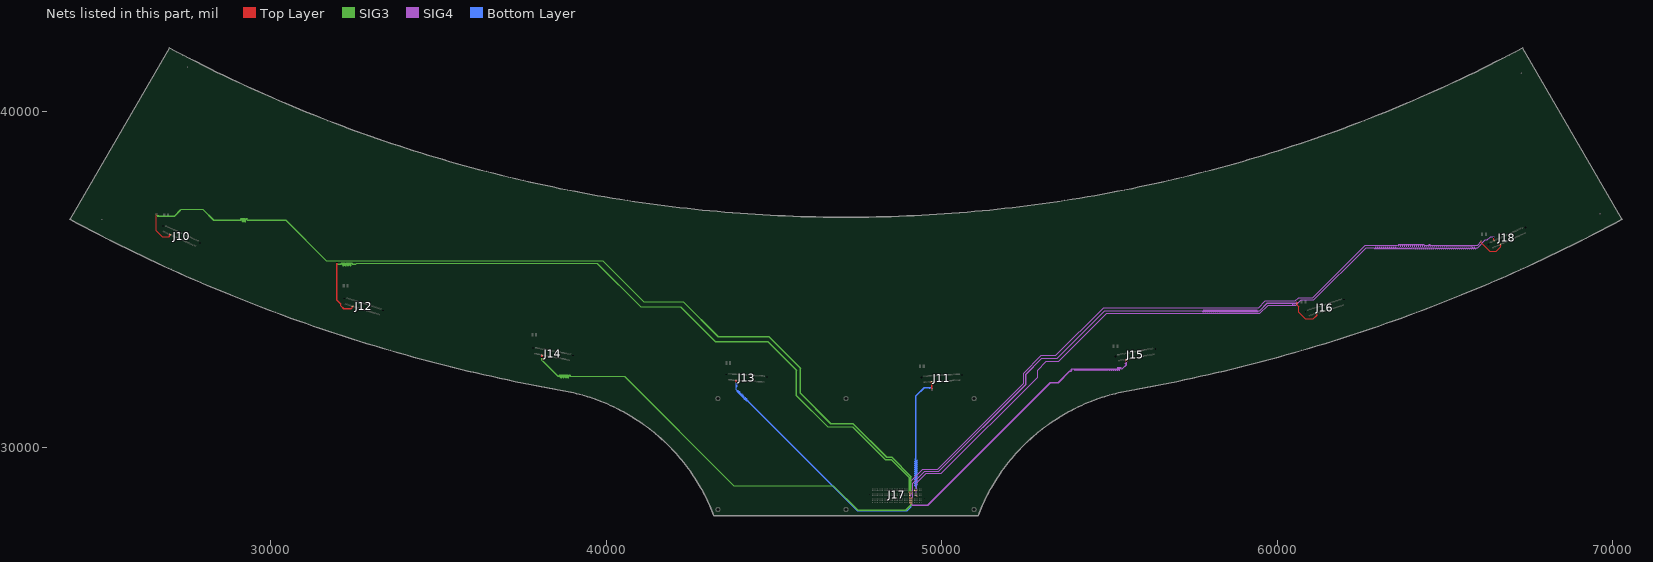
[diagram p0: the nets of this part, all layers, seen from the top]
# Altium PCB MISC86329.PcbDoc (part 3 of 11)
Units mil, origin at the board's own origin, x right, y up, seen from the top; angles counter-clockwise.
Board outline 46247.15 x 13937.21 mil, 6 copper layers (Top Layer, GND2, SIG3, SIG4, POWER5, Bottom Layer); 17 components, 210 nets, 908 pads, 1109 vias.

## Via types
v1: diameter 24, hole 12, Top Layer to Bottom Layer, 684 vias
v2: diameter 18, hole 9, Top Layer to Bottom Layer, 425 vias

## Nets (pads, with @x,y where several pads share a name; then routed paths per layer and width w, separated by ;. In a path a pad name is that pad's centre, name@x,y a point inside that pad or via, vN(x,y) a via of type N, cw(c..) or ccw(c..) an arc to the next point about the centre after c; other vN are vias at no path point) (continued)
DATAIN0P_CH7: J17.E4 J18.10 | length 23895.7
  Top Layer w5: J17.E4@49237.89,28568.8 v2(49261.69,28545) ; v2(66447.5,36256) 66454,36249.5 66454,36196.31 66459.31,36191 J18.10@66459.31,36164.1
  SIG4 w5: v2(49261.69,28545) 49241.69,28565 49241.69,28940.55 49534.14,29233 49992.14,29233 52860,32100.86 52860,32310 53122,32572 53491.14,32572 54914.14,33995 59484.14,33995 59729.14,34240 60552.14,34240 60712.14,34400 61087.14,34400 62648.14,35961 62884.43,35961 62889,35956.43 62889,35941.43 62899.43,35931 62918.57,35931 62929,35941.43 62929,35986.43 62933.57,35991 62944.43,35991 62949,35986.43 62949,35941.43 62959.43,35931 62978.57,35931 62989,35941.43 62989,35986.43 62993.57,35991 63004.43,35991 63009,35986.43 63009,35941.43 63019.43,35931 63038.57,35931 63049,35941.43 63049,35986.43 63053.57,35991 63064.43,35991 63069,35986.43 63069,35941.43 63079.43,35931 63098.57,35931 63109,35941.43 63109,35986.43 63113.57,35991 63124.43,35991 63129,35986.43 63129,35941.43 63139.43,35931 63158.57,35931 63169,35941.43 63169,35986.43 63173.57,35991 63184.43,35991 63189,35986.43 63189,35941.43 63199.43,35931 63218.57,35931 63229,35941.43 63229,35986.43 63233.57,35991 63244.43,35991 63249,35986.43 63249,35941.43 63259.43,35931 63278.57,35931 63289,35941.43 63289,35986.43 63293.57,35991 63304.43,35991 63309,35986.43 63309,35941.43 63319.43,35931 63338.57,35931 63349,35941.43 63349,35986.43 63353.57,35991 63364.43,35991 63369,35986.43 63369,35941.43 63379.43,35931 63398.57,35931 63409,35941.43 63409,35986.43 63413.57,35991 63424.43,35991 63429,35986.43 63429,35941.43 63439.43,35931 63458.57,35931 63469,35941.43 63469,35986.43 63473.57,35991 63484.43,35991 63489,35986.43 63489,35941.43 63499.43,35931 63518.57,35931 63529,35941.43 63529,35986.43 63533.57,35991 63544.43,35991 63549,35986.43 63549,35941.43 63559.43,35931 63578.57,35931 63589,35941.43 63589,35956.43 63593.57,35961 63604.43,35961 63609,35956.43 63609,35941.43 63619.43,35931 63638.57,35931 63649,35941.43 63649,35956.43 63653.57,35961 63664.43,35961 63669,35956.43 63669,35941.43 63679.43,35931 63698.57,35931 63709,35941.43 63709,35956.43 63713.57,35961 63724.43,35961 63729,35956.43 63729,35941.43 63739.43,35931 63758.57,35931 63769,35941.43 63769,35956.43 63773.57,35961 63784.43,35961 63789,35956.43 63789,35941.43 63799.43,35931 63818.57,35931 63829,35941.43 63829,35956.43 63833.57,35961 63844.43,35961 63849,35956.43 63849,35941.43 63859.43,35931 63878.57,35931 63889,35941.43 63889,35956.43 63893.57,35961 63904.43,35961 63909,35956.43 63909,35941.43 63919.43,35931 63938.57,35931 63949,35941.43 63949,35956.43 63953.57,35961 63964.43,35961 63969,35956.43 63969,35941.43 63979.43,35931 63998.57,35931 64009,35941.43 64009,35956.43 64013.57,35961 64024.43,35961 64029,35956.43 64029,35941.43 64039.43,35931 64058.57,35931 64069,35941.43 64069,35956.43 64073.57,35961 64084.43,35961 64089,35956.43 64089,35941.43 64099.43,35931 64118.57,35931 64129,35941.43 64129,35956.43 64133.57,35961 64144.43,35961 64149,35956.43 64149,35941.43 64159.43,35931 64178.57,35931 64189,35941.43 64189,35956.43 64193.57,35961 64204.43,35961 64209,35956.43 64209,35941.43 64219.43,35931 64238.57,35931 64249,35941.43 64249,35956.43 64253.57,35961 64264.43,35961 64269,35956.43 64269,35941.43 64279.43,35931 64298.57,35931 64309,35941.43 64309,35956.43 64313.57,35961 64324.43,35961 64329,35956.43 64329,35941.43 64339.43,35931 64358.57,35931 64369,35941.43 64369,35956.43 64373.57,35961 64384.43,35961 64389,35956.43 64389,35941.43 64399.43,35931 64418.57,35931 64429,35941.43 64429,35956.43 64433.57,35961 64444.43,35961 64449,35956.43 64449,35941.43 64459.43,35931 64478.57,35931 64489,35941.43 64489,35956.43 64493.57,35961 64504.43,35961 64509,35956.43 64509,35941.43 64519.43,35931 64538.57,35931 64549,35941.43 64549,35956.43 64553.57,35961 64564.43,35961 64569,35956.43 64569,35941.43 64579.43,35931 64598.57,35931 64609,35941.43 64609,35956.43 64613.57,35961 64624.43,35961 64629,35956.43 64629,35941.43 64639.43,35931 64658.57,35931 64669,35941.43 64669,35956.43 64673.57,35961 64684.43,35961 64689,35956.43 64689,35941.43 64699.43,35931 64718.57,35931 64729,35941.43 64729,35956.43 64733.57,35961 64744.43,35961 64749,35956.43 64749,35941.43 64759.43,35931 64778.57,35931 64789,35941.43 64789,35956.43 64793.57,35961 64804.43,35961 64809,35956.43 64809,35941.43 64819.43,35931 64838.57,35931 64849,35941.43 64849,35956.43 64853.57,35961 64864.43,35961 64869,35956.43 64869,35941.43 64879.43,35931 64898.57,35931 64909,35941.43 64909,35956.43 64913.57,35961 64924.43,35961 64929,35956.43 64929,35941.43 64939.43,35931 64958.57,35931 64969,35941.43 64969,35956.43 64973.57,35961 64984.43,35961 64989,35956.43 64989,35941.43 64999.43,35931 65018.57,35931 65029,35941.43 65029,35956.43 65033.57,35961 65044.43,35961 65049,35956.43 65049,35941.43 65059.43,35931 65078.57,35931 65089,35941.43 65089,35956.43 65093.57,35961 65104.43,35961 65109,35956.43 65109,35941.43 65119.43,35931 65138.57,35931 65149,35941.43 65149,35956.43 65153.57,35961 65164.43,35961 65169,35956.43 65169,35941.43 65179.43,35931 65198.57,35931 65209,35941.43 65209,35956.43 65213.57,35961 65224.43,35961 65229,35956.43 65229,35941.43 65239.43,35931 65258.57,35931 65269,35941.43 65269,35956.43 65273.57,35961 65284.43,35961 65289,35956.43 65289,35941.43 65299.43,35931 65318.57,35931 65329,35941.43 65329,35956.43 65333.57,35961 65344.43,35961 65349,35956.43 65349,35941.43 65359.43,35931 65378.57,35931 65389,35941.43 65389,35956.43 65393.57,35961 65404.43,35961 65409,35956.43 65409,35941.43 65419.43,35931 65438.57,35931 65449,35941.43 65449,35956.43 65453.57,35961 65464.43,35961 65469,35956.43 65469,35941.43 65479.43,35931 65498.57,35931 65509,35941.43 65509,35956.43 65513.57,35961 65524.43,35961 65529,35956.43 65529,35941.43 65539.43,35931 65558.57,35931 65569,35941.43 65569,35956.43 65573.57,35961 65584.43,35961 65589,35956.43 65589,35941.43 65599.43,35931 65618.57,35931 65629,35941.43 65629,35956.43 65633.57,35961 65644.43,35961 65649,35956.43 65649,35941.43 65659.43,35931 65678.57,35931 65689,35941.43 65689,35956.43 65693.57,35961 65704.43,35961 65709,35956.43 65709,35941.43 65719.43,35931 65738.57,35931 65749,35941.43 65749,35956.43 65753.57,35961 65764.43,35961 65769,35956.43 65769,35941.43 65779.43,35931 65798.57,35931 65809,35941.43 65809,35986.43 65813.57,35991 65824.43,35991 65829,35986.43 65829,35941.43 65839.43,35931 65858.57,35931 65869,35941.43 65869,35986.43 65873.57,35991 65884.43,35991 65889,35986.43 65889,35941.43 65899.43,35931 65918.57,35931 65929,35941.43 65929,35956.43 65933.57,35961 65966.14,35961 66200.14,36195 66263.14,36195 66354.14,36286 66395,36286 66398,36283 66398,36277.73 66401,36274.73 66415,36274.73 66418,36277.73 66418,36283 66421,36286 66442.86,36286 66455,36273.86 66455,36265 v2@66448,36258
DATAIN1N_CH0: J10.17 J17.G8 | length 28225.1
  Top Layer w5: v2(26587.5,36961) 26594,36954.5 26594,36458.86 26773.86,36279 26978.14,36279 27033.49,36334.35 J10.17@27033.49,36336.19 ; J17.G8@49037.89,28668.8 v2(49061.69,28692.61)
  SIG3 w5: v2(26587.5,36961) 26594,36954.5 26594,36925.86 26621.86,36898 27146.14,36898 27323.57,37075.43 ; 27324.07,37075.93 27323.57,37075.43 ; 27359,37098 27362,37098 ; v2(49061.69,28692.61) 49081.69,28712.61 49081.69,29133.31 48505,29710 48351.86,29710 47345.86,30716 46683.86,30716 45787,31612.86 45787,32360 44841,33306 43332.86,33306 42297.86,34341 41116.86,34341 39896.86,35561 31663.86,35561 30448.86,36776 29307.18,36776 29295.5,36787.68 29295.5,36810.18 29289.68,36816 29276.32,36816 29270.5,36810.18 29270.5,36747.68 29258.82,36736 29237.18,36736 29225.5,36747.68 29225.5,36810.18 29219.68,36816 29206.32,36816 29200.5,36810.18 29200.5,36747.68 29188.82,36736 29167.18,36736 29155.5,36747.68 29155.5,36810.18 29149.68,36816 29136.32,36816 29130.5,36810.18 29130.5,36787.68 29118.82,36776 28298.86,36776 27976.86,37098 27362,37098 ; 27323.57,37075.43 27346.14,37098 27362,37098
DATAIN1N_CH1: J12.17 J17.F8 | length 23094.8
  Top Layer w5: 31975,35509.5 31975,34386.86 32088,34273.86 32088,34219.86 32172.86,34135 32410.14,34135 32442.98,34167.84 32442.98,34187.61 J12.17@32463.01,34207.64 ; J17.F8@49037.89,28618.8 v2(49061.69,28642.61)
  SIG3 w5: v2(31968.5,35516) v2@31971,35516 ; v2@31970,35517 v2@31971,35516 ; v2@31975,35516 v2@31971,35516 ; v2(49061.69,28642.61) 49032,28672.3 49032,29102 48492,29642 48312.86,29642 47341.86,30613 46603.86,30613 45673,31543.86 45673,32302 44819,33156 43248.86,33156 42215.86,34189 41027.86,34189 39728.86,35488 32571.14,35488 32545.14,35462 32441.18,35462 32429.5,35473.68 32429.5,35494.91 32423.68,35500.73 32410.32,35500.73 32404.5,35494.91 32404.5,35434.95 32392.82,35423.27 32371.18,35423.27 32359.5,35434.95 32359.5,35494.91 32353.68,35500.73 32340.32,35500.73 32334.5,35494.91 32334.5,35434.95 32322.82,35423.27 32301.18,35423.27 32289.5,35434.95 32289.5,35494.91 32283.68,35500.73 32270.32,35500.73 32264.5,35494.91 32264.5,35434.95 32252.82,35423.27 32231.18,35423.27 32219.5,35434.95 32219.5,35494.91 32213.68,35500.73 32200.32,35500.73 32194.5,35494.91 32194.5,35434.95 32182.82,35423.27 32161.18,35423.27 32149.5,35434.95 32149.5,35494.91 32143.68,35500.73 32130.32,35500.73 32124.5,35494.91 32124.5,35473.68 32112.82,35462 31999,35462 31975,35486 31975,35512 v2@31971,35516
DATAIN1N_CH2: J14.17 J17.B8 | length 13805.5
  Top Layer w5: v2(38103.5,32687) 38097,32693.5 38097,32728 38110,32741 J14.17@38110,32753 ; J14.17@38111.46,32753 J14.17@38111.46,32756.64 ; J17.B8@49037.89,28418.8 v2(49061.69,28395)
  SIG3 w5: v2@38103,32685 38097,32679 38097,32662.75 38103.25,32656.5 38115.92,32656.5 38122.17,32650.25 38122.17,32637.75 38115.92,32631.5 38103.25,32631.5 38097,32625.25 38097,32599 38568,32128 38598.68,32128 38604.5,32133.82 38604.5,32153.32 38616.18,32165 38637.82,32165 38649.5,32153.32 38649.5,32096.82 38655.32,32091 38668.68,32091 38674.5,32096.82 38674.5,32153.32 38686.18,32165 38707.82,32165 38719.5,32153.32 38719.5,32096.82 38725.32,32091 38738.68,32091 38744.5,32096.82 38744.5,32153.32 38756.18,32165 38777.82,32165 38789.5,32153.32 38789.5,32096.82 38795.32,32091 38808.68,32091 38814.5,32096.82 38814.5,32153.32 38826.18,32165 38847.82,32165 38859.5,32153.32 38859.5,32096.82 38865.32,32091 38878.68,32091 38884.5,32096.82 38884.5,32153.32 38896.18,32165 38917.82,32165 38929.5,32153.32 38929.5,32133.82 38935.32,32128 40551,32128 43810,28869 46771,28869 47499,28141 48933,28141 49081.69,28289.69 49081.69,28375 v2(49061.69,28395)
DATAIN1N_CH3: J13.17 J17.A8 | length 7748.3
  Top Layer w5: 43883.92,31946.5 43883.92,31969.28 43894.64,31980 J13.17@43894.64,32004.84 ; J17.A8@49037.89,28368.8 v2(49061.69,28345)
  Bottom Layer w5: v2@43889,31937 43884,31932 43884,31898.5 43889,31893.5 43896.36,31893.5 43901.36,31888.5 43901.36,31873.5 43896.36,31868.5 43889,31868.5 43884,31863.5 43884,31848.5 43889,31843.5 43896.36,31843.5 43901.36,31838.5 43901.36,31823.5 43896.36,31818.5 43889,31818.5 43884,31813.5 43884,31729 43906.95,31706.05 43911.65,31706.05 43916.95,31711.35 43929.94,31711.35 43941.7,31699.58 43941.7,31686.6 43922.26,31667.15 43922.26,31662.46 43928.17,31656.55 43932.86,31656.55 43952.31,31675.99 43965.29,31675.99 43977.06,31664.23 43977.06,31651.24 43957.61,31631.8 43957.61,31627.1 43963.52,31621.19 43968.22,31621.19 43987.67,31640.64 44000.65,31640.64 44012.41,31628.87 44012.41,31615.89 43992.97,31596.44 43992.97,31591.75 43998.88,31585.84 44003.58,31585.84 44023.02,31605.28 44036,31605.28 44047.77,31593.51 44047.77,31580.53 44028.32,31561.09 44028.32,31556.39 44034.23,31550.48 44038.93,31550.48 44058.38,31569.93 44071.36,31569.93 44083.12,31558.16 44083.12,31545.18 44063.68,31525.73 44063.68,31521.04 44069.59,31515.13 44074.29,31515.13 44093.73,31534.57 44106.71,31534.57 44118.48,31522.8 44118.48,31509.82 44099.03,31490.38 44099.03,31485.68 44104.94,31479.77 44109.64,31479.77 44129.09,31499.22 44142.07,31499.22 44153.84,31487.45 44153.84,31474.47 44134.39,31455.02 44134.39,31450.33 44140.3,31444.42 44145,31444.42 44164.44,31463.86 44177.42,31463.86 44189.19,31452.09 44189.19,31439.11 44169.75,31419.67 44169.75,31414.97 44175.66,31409.06 44180.35,31409.06 44199.8,31428.51 44212.78,31428.51 44224.55,31416.74 44224.55,31403.76 44219.24,31398.45 44219.24,31393.76 47481,28132 48977,28132 49081.69,28236.69 49081.69,28325 v2(49061.69,28345)
  other v2: 43890.42,31940
DATAIN1N_CH4: J11.17 J17.H5 | length 5093.3
  Top Layer w5: J17.H5@49187.89,28718.8 v2(49211.69,28742.61) ; 49715.61,31718.5 49715.61,31927.28 49726.33,31938 J11.17@49726.33,31963.43
  Bottom Layer w5: v2(49211.69,28742.61) 49231.69,28762.61 49231.69,28842.43 49227.12,28847 49212.12,28847 49201.69,28857.43 49201.69,28876.57 49212.12,28887 49257.12,28887 49261.69,28891.57 49261.69,28902.43 49257.12,28907 49212.12,28907 49201.69,28917.43 49201.69,28936.57 49212.12,28947 49257.12,28947 49261.69,28951.57 49261.69,28962.43 49257.12,28967 49212.12,28967 49201.69,28977.43 49201.69,28996.57 49212.12,29007 49257.12,29007 49261.69,29011.57 49261.69,29022.43 49257.12,29027 49212.12,29027 49201.69,29037.43 49201.69,29056.57 49212.12,29067 49257.12,29067 49261.69,29071.57 49261.69,29082.43 49257.12,29087 49212.12,29087 49201.69,29097.43 49201.69,29116.57 49212.12,29127 49257.12,29127 49261.69,29131.57 49261.69,29142.43 49257.12,29147 49212.12,29147 49201.69,29157.43 49201.69,29176.57 49212.12,29187 49257.12,29187 49261.69,29191.57 49261.69,29202.43 49257.12,29207 49212.12,29207 49201.69,29217.43 49201.69,29236.57 49212.12,29247 49257.12,29247 49261.69,29251.57 49261.69,29262.43 49257.12,29267 49212.12,29267 49201.69,29277.43 49201.69,29296.57 49212.12,29307 49257.12,29307 49261.69,29311.57 49261.69,29322.43 49257.12,29327 49212.12,29327 49201.69,29337.43 49201.69,29356.57 49212.12,29367 49257.12,29367 49261.69,29371.57 49261.69,29382.43 49257.12,29387 49212.12,29387 49201.69,29397.43 49201.69,29416.57 49212.12,29427 49257.12,29427 49261.69,29431.57 49261.69,29442.43 49257.12,29447 49212.12,29447 49201.69,29457.43 49201.69,29476.57 49212.12,29487 49257.12,29487 49261.69,29491.57 49261.69,29502.43 49257.12,29507 49212.12,29507 49201.69,29517.43 49201.69,29536.57 49212.12,29547 49257.12,29547 49261.69,29551.57 49261.69,29562.43 49257.12,29567 49212.12,29567 49201.69,29577.43 49201.69,29596.57 49212.12,29607 49257.12,29607 49261.69,29611.57 49261.69,29622.43 49257.12,29627 49227,29627 49214,29640 49214,29669.14 49231.69,29686.83 49231.69,31545.69 49485,31799 49672.14,31799 49716,31755.14 49716,31717 v2@49721,31712
  other v2: 49722.11,31712
DATAIN1N_CH5: J15.17 J17.C8 | length 10127.3
  Top Layer w5: J17.C8@49037.89,28468.8 v2(49061.69,28445) ; v2(55513.5,32564) 55507,32570.5 55507,32594.39 55519.61,32607 J15.17@55519.61,32633.03
  SIG4 w5: v2(49061.69,28445) 49081.69,28425 49081.69,28330.17 49125.86,28286 49595.14,28286 53246.14,31937 53481.14,31937 53822.14,32278 53853.29,32278 ; 53853.32,32277.97 53867.97,32277.97 53880,32290 53880,32307.86 53874.54,32313.32 53874.54,32330.39 53887.14,32343 53946.43,32343 53951,32338.43 53951,32313.43 53961.43,32303 53980.57,32303 53991,32313.43 53991,32338.43 53995.57,32343 54006.43,32343 54011,32338.43 54011,32313.43 54021.43,32303 54040.57,32303 54051,32313.43 54051,32338.43 54055.57,32343 54066.43,32343 54071,32338.43 54071,32313.43 54081.43,32303 54100.57,32303 54111,32313.43 54111,32338.43 54115.57,32343 54126.43,32343 54131,32338.43 54131,32313.43 54141.43,32303 54160.57,32303 54171,32313.43 54171,32338.43 54175.57,32343 54186.43,32343 54191,32338.43 54191,32313.43 54201.43,32303 54220.57,32303 54231,32313.43 54231,32338.43 54235.57,32343 54246.43,32343 54251,32338.43 54251,32313.43 54261.43,32303 54280.57,32303 54291,32313.43 54291,32338.43 54295.57,32343 54306.43,32343 54311,32338.43 54311,32313.43 54321.43,32303 54340.57,32303 54351,32313.43 54351,32338.43 54355.57,32343 54366.43,32343 54371,32338.43 54371,32313.43 54381.43,32303 54400.57,32303 54411,32313.43 54411,32338.43 54415.57,32343 54426.43,32343 54431,32338.43 54431,32313.43 54441.43,32303 54460.57,32303 54471,32313.43 54471,32338.43 54475.57,32343 54486.43,32343 54491,32338.43 54491,32313.43 54501.43,32303 54520.57,32303 54531,32313.43 54531,32338.43 54535.57,32343 54546.43,32343 54551,32338.43 54551,32313.43 54561.43,32303 54580.57,32303 54591,32313.43 54591,32338.43 54595.57,32343 54606.43,32343 54611,32338.43 54611,32313.43 54621.43,32303 54640.57,32303 54651,32313.43 54651,32338.43 54655.57,32343 54666.43,32343 54671,32338.43 54671,32313.43 54681.43,32303 54700.57,32303 54711,32313.43 54711,32338.43 54715.57,32343 54726.43,32343 54731,32338.43 54731,32313.43 54741.43,32303 54760.57,32303 54771,32313.43 54771,32338.43 54775.57,32343 54786.43,32343 54791,32338.43 54791,32313.43 54801.43,32303 54820.57,32303 54831,32313.43 54831,32338.43 54835.57,32343 54846.43,32343 54851,32338.43 54851,32313.43 54861.43,32303 54880.57,32303 54891,32313.43 54891,32338.43 54895.57,32343 54906.43,32343 54911,32338.43 54911,32313.43 54921.43,32303 54940.57,32303 54951,32313.43 54951,32338.43 54955.57,32343 54966.43,32343 54971,32338.43 54971,32313.43 54981.43,32303 55000.57,32303 55011,32313.43 55011,32338.43 55015.57,32343 55026.43,32343 55031,32338.43 55031,32313.43 55041.43,32303 55060.57,32303 55071,32313.43 55071,32338.43 55075.57,32343 55086.43,32343 55091,32338.43 55091,32313.43 55101.43,32303 55120.57,32303 55131,32313.43 55131,32338.43 55135.57,32343 55146.43,32343 55151,32338.43 55151,32313.43 55161.43,32303 55180.57,32303 55191,32313.43 55191,32338.43 55195.57,32343 55206.43,32343 55211,32338.43 55211,32313.43 55221.43,32303 55240.57,32303 55251,32313.43 55251,32378.43 55255.57,32383 55266.43,32383 55271,32378.43 55271,32313.43 55281.43,32303 55300.57,32303 55311,32313.43 55311,32378.43 55315.57,32383 55326.43,32383 55331,32378.43 55331,32353.43 55341.43,32343 55382,32343 55507,32468 55507,32556 v2@55515,32564
DATAIN1N_CH6: J16.17 J17.D8 | length 18293.4
  Top Layer w5: J17.D8@49037.89,28518.8 v2(49061.69,28495) ; 60590,34344.5 60590,34240 60634,34196 60634,34030.86 60832.86,33832 61077.14,33832 61187,33941.86 61187,33975.91 ; 61188.09,33977 J16.17@61188.09,34003.67
  SIG4 w5: v2(49061.69,28495) 49088.36,28495 49104.86,28511.5 49113.5,28511.5 49131,28529 49131,28937 49492,29298 49914,29298 52506,31890 52506,32186.14 52984.86,32665 53444,32665 54860,34081 57770,34081 57783,34068 57783,34055.57 57787.57,34051 57798.43,34051 57803,34055.57 57803,34100.57 57813.43,34111 57832.57,34111 57843,34100.57 57843,34055.57 57847.57,34051 57858.43,34051 57863,34055.57 57863,34100.57 57873.43,34111 57892.57,34111 57903,34100.57 57903,34055.57 57907.57,34051 57918.43,34051 57923,34055.57 57923,34100.57 57933.43,34111 57952.57,34111 57963,34100.57 57963,34055.57 57967.57,34051 57978.43,34051 57983,34055.57 57983,34100.57 57993.43,34111 58012.57,34111 58023,34100.57 58023,34055.57 58027.57,34051 58038.43,34051 58043,34055.57 58043,34100.57 58053.43,34111 58072.57,34111 58083,34100.57 58083,34055.57 58087.57,34051 58098.43,34051 58103,34055.57 58103,34100.57 58113.43,34111 58132.57,34111 58143,34100.57 58143,34055.57 58147.57,34051 58158.43,34051 58163,34055.57 58163,34100.57 58173.43,34111 58192.57,34111 58203,34100.57 58203,34055.57 58207.57,34051 58218.43,34051 58223,34055.57 58223,34100.57 58233.43,34111 58252.57,34111 58263,34100.57 58263,34055.57 58267.57,34051 58278.43,34051 58283,34055.57 58283,34100.57 58293.43,34111 58312.57,34111 58323,34100.57 58323,34055.57 58327.57,34051 58338.43,34051 58343,34055.57 58343,34100.57 58353.43,34111 58372.57,34111 58383,34100.57 58383,34055.57 58387.57,34051 58398.43,34051 58403,34055.57 58403,34100.57 58413.43,34111 58432.57,34111 58443,34100.57 58443,34055.57 58447.57,34051 58458.43,34051 58463,34055.57 58463,34100.57 58473.43,34111 58492.57,34111 58503,34100.57 58503,34055.57 58507.57,34051 58518.43,34051 58523,34055.57 58523,34100.57 58533.43,34111 58552.57,34111 58563,34100.57 58563,34055.57 58567.57,34051 58578.43,34051 58583,34055.57 58583,34100.57 58593.43,34111 58612.57,34111 58623,34100.57 58623,34055.57 58627.57,34051 58638.43,34051 58643,34055.57 58643,34100.57 58653.43,34111 58672.57,34111 58683,34100.57 58683,34055.57 58687.57,34051 58698.43,34051 58703,34055.57 58703,34100.57 58713.43,34111 58732.57,34111 58743,34100.57 58743,34055.57 58747.57,34051 58758.43,34051 58763,34055.57 58763,34100.57 58773.43,34111 58792.57,34111 58803,34100.57 58803,34055.57 58807.57,34051 58818.43,34051 58823,34055.57 58823,34100.57 58833.43,34111 58852.57,34111 58863,34100.57 58863,34055.57 58867.57,34051 58878.43,34051 58883,34055.57 58883,34100.57 58893.43,34111 58912.57,34111 58923,34100.57 58923,34055.57 58927.57,34051 58938.43,34051 58943,34055.57 58943,34100.57 58953.43,34111 58972.57,34111 58983,34100.57 58983,34055.57 58987.57,34051 58998.43,34051 59003,34055.57 59003,34100.57 59013.43,34111 59032.57,34111 59043,34100.57 59043,34055.57 59047.57,34051 59058.43,34051 59063,34055.57 59063,34100.57 59073.43,34111 59092.57,34111 59103,34100.57 59103,34055.57 59107.57,34051 59118.43,34051 59123,34055.57 59123,34100.57 59133.43,34111 59152.57,34111 59163,34100.57 59163,34055.57 59167.57,34051 59178.43,34051 59183,34055.57 59183,34100.57 59193.43,34111 59212.57,34111 59223,34100.57 59223,34055.57 59227.57,34051 59238.43,34051 59243,34055.57 59243,34100.57 59253.43,34111 59272.57,34111 59283,34100.57 59283,34055.57 59287.57,34051 59298.43,34051 59303,34055.57 59303,34100.57 59313.43,34111 59332.57,34111 59343,34100.57 59343,34055.57 59347.57,34051 59358.43,34051 59363,34055.57 59363,34100.57 59373.43,34111 59392.57,34111 59403,34100.57 59403,34055.57 59407.57,34051 59418.43,34051 59423,34055.57 59423,34070.57 59433.43,34081 59472,34081 59699,34308 60564,34308 60590,34334 60590,34346 v2@60584,34352
  other v2: 60583.5,34351
DATAIN1N_CH7: J17.E8 J18.17 | length 23896.2
  Top Layer w5: J17.E8@49037.89,28568.8 v2(49061.69,28545) ; 66083,36150.5 66083,36099.86 66328.86,35854 66531.14,35854 66654,35976.86 66654,36020.63 66647.29,36027.34 J18.17@66647.29,36054.9
  SIG4 w5: v2(49061.69,28545) 49081.69,28565 49081.69,29002.14 49440.55,29361 49888,29361 52438,31911 52438,32218 52965,32745 53404,32745 54828,34169 59448,34169 59647,34368 60538,34368 60636,34466 61051,34466 62619,36034 63576,36034 63599,36011 63612,36011 63621.5,36020.5 63621.5,36053.57 63631.93,36064 63651.07,36064 63661.5,36053.57 63661.5,36008.57 63666.07,36004 63676.93,36004 63681.5,36008.57 63681.5,36053.57 63691.93,36064 63711.07,36064 63721.5,36053.57 63721.5,36008.57 63726.07,36004 63736.93,36004 63741.5,36008.57 63741.5,36053.57 63751.93,36064 63771.07,36064 63781.5,36053.57 63781.5,36008.57 63786.07,36004 63796.93,36004 63801.5,36008.57 63801.5,36053.57 63811.93,36064 63831.07,36064 63841.5,36053.57 63841.5,36008.57 63846.07,36004 63856.93,36004 63861.5,36008.57 63861.5,36053.57 63871.93,36064 63891.07,36064 63901.5,36053.57 63901.5,36008.57 63906.07,36004 63916.93,36004 63921.5,36008.57 63921.5,36053.57 63931.93,36064 63951.07,36064 63961.5,36053.57 63961.5,36008.57 63966.07,36004 63976.93,36004 63981.5,36008.57 63981.5,36053.57 63991.93,36064 64011.07,36064 64021.5,36053.57 64021.5,36008.57 64026.07,36004 64036.93,36004 64041.5,36008.57 64041.5,36053.57 64051.93,36064 64071.07,36064 64081.5,36053.57 64081.5,36008.57 64086.07,36004 64096.93,36004 64101.5,36008.57 64101.5,36053.57 64111.93,36064 64131.07,36064 64141.5,36053.57 64141.5,36008.57 64146.07,36004 64156.93,36004 64161.5,36008.57 64161.5,36053.57 64171.93,36064 64191.07,36064 64201.5,36053.57 64201.5,36008.57 64206.07,36004 64216.93,36004 64221.5,36008.57 64221.5,36053.57 64231.93,36064 64251.07,36064 64261.5,36053.57 64261.5,36008.57 64266.07,36004 64276.93,36004 64281.5,36008.57 64281.5,36053.57 64291.93,36064 64311.07,36064 64321.5,36053.57 64321.5,36008.57 64326.07,36004 64336.93,36004 64341.5,36008.57 64341.5,36053.57 64351.93,36064 64371.07,36064 64381.5,36053.57 64381.5,36008.57 64386.07,36004 64396.93,36004 64401.5,36008.57 64401.5,36023.57 64411.93,36034 64431.07,36034 64441.5,36023.57 64441.5,36008.57 64446.07,36004 64456.93,36004 64461.5,36008.57 64461.5,36023.57 64471.93,36034 64491.07,36034 64501.5,36023.57 64501.5,36008.57 64506.07,36004 64516.93,36004 64521.5,36008.57 64521.5,36053.57 64531.93,36064 64551.07,36064 64561.5,36053.57 64561.5,36008.57 64566.07,36004 64576.93,36004 64581.5,36008.57 64581.5,36023.57 64591.93,36034 64611.07,36034 64621.5,36023.57 64621.5,36008.57 64626.07,36004 64636.93,36004 64641.5,36008.57 64641.5,36023.57 64651.93,36034 64671.07,36034 64681.5,36023.57 64681.5,36008.57 64686.07,36004 64696.93,36004 64701.5,36008.57 64701.5,36023.57 64711.93,36034 64731.07,36034 64741.5,36023.57 64741.5,36008.57 64746.07,36004 64756.93,36004 64761.5,36008.57 64761.5,36023.57 64771.93,36034 64791.07,36034 64801.5,36023.57 64801.5,36008.57 64806.07,36004 64816.93,36004 64821.5,36008.57 64821.5,36023.57 64831.93,36034 64851.07,36034 64861.5,36023.57 64861.5,36008.57 64866.07,36004 64876.93,36004 64881.5,36008.57 64881.5,36023.57 64891.93,36034 64911.07,36034 64921.5,36023.57 64921.5,36008.57 64926.07,36004 64936.93,36004 64941.5,36008.57 64941.5,36023.57 64951.93,36034 64971.07,36034 64981.5,36023.57 64981.5,36008.57 64986.07,36004 64996.93,36004 65001.5,36008.57 65001.5,36023.57 65011.93,36034 65031.07,36034 65041.5,36023.57 65041.5,36008.57 65046.07,36004 65056.93,36004 65061.5,36008.57 65061.5,36023.57 65071.93,36034 65091.07,36034 65101.5,36023.57 65101.5,36008.57 65106.07,36004 65116.93,36004 65121.5,36008.57 65121.5,36023.57 65131.93,36034 65151.07,36034 65161.5,36023.57 65161.5,36008.57 65166.07,36004 65176.93,36004 65181.5,36008.57 65181.5,36023.57 65191.93,36034 65211.07,36034 65221.5,36023.57 65221.5,36008.57 65226.07,36004 65236.93,36004 65241.5,36008.57 65241.5,36023.57 65251.93,36034 65271.07,36034 65281.5,36023.57 65281.5,36008.57 65286.07,36004 65296.93,36004 65301.5,36008.57 65301.5,36023.57 65311.93,36034 65331.07,36034 65341.5,36023.57 65341.5,36008.57 65346.07,36004 65356.93,36004 65361.5,36008.57 65361.5,36023.57 65371.93,36034 65391.07,36034 65401.5,36023.57 65401.5,36008.57 65406.07,36004 65416.93,36004 65421.5,36008.57 65421.5,36023.57 65431.93,36034 65451.07,36034 65461.5,36023.57 65461.5,36008.57 65466.07,36004 65476.93,36004 65481.5,36008.57 65481.5,36023.57 65491.93,36034 65511.07,36034 65521.5,36023.57 65521.5,36008.57 65526.07,36004 65536.93,36004 65541.5,36008.57 65541.5,36023.57 65551.93,36034 65571.07,36034 65581.5,36023.57 65581.5,36008.57 65586.07,36004 65596.93,36004 65601.5,36008.57 65601.5,36023.57 65611.93,36034 65631.07,36034 65641.5,36023.57 65641.5,36008.57 65646.07,36004 65656.93,36004 65661.5,36008.57 65661.5,36023.57 65671.93,36034 65691.07,36034 65701.5,36023.57 65701.5,36008.57 65706.07,36004 65716.93,36004 65721.5,36008.57 65721.5,36023.57 65731.93,36034 65751.07,36034 65761.5,36023.57 65761.5,36008.57 65766.07,36004 65776.93,36004 65781.5,36008.57 65781.5,36023.57 65791.93,36034 65975.86,36034 66083,36141.14 66083,36151 v2@66079,36155
  other v2: 66076.5,36157
DATAIN1P_CH0: J10.15 J17.G7 | length 28224.5
  Top Layer w5: v2(26610.5,36961) 26604,36954.5 26604,36463 26778,36289 26974,36289 27004.85,36319.85 J10.15@27004.85,36349.28 ; J17.G7@49087.89,28668.8 v2(49111.69,28692.61)
  SIG3 w5: v2(26610.5,36961) 26604,36954.5 26604,36930 26626,36908 26652,36908 26657,36913 26657,36921.38 26662,36926.38 26672,36926.38 26677,36921.38 26677,36913 26682,36908 27142,36908 27315,37081 ; 27317,37083 27315,37081 ; 27359,37108 27362,37108 ; v2(49111.69,28692.61) 49091.69,28712.61 49091.69,29137.45 48509.14,29720 48356,29720 47350,30726 46688,30726 45797,31617 45797,32364.14 44845.14,33316 43337,33316 42302,34351 41121,34351 39901,35571 31668,35571 30453,36786 29311.32,36786 29305.5,36791.82 29305.5,36814.32 29293.82,36826 29272.18,36826 29260.5,36814.32 29260.5,36751.82 29254.68,36746 29241.32,36746 29235.5,36751.82 29235.5,36814.32 29223.82,36826 29202.18,36826 29190.5,36814.32 29190.5,36751.82 29184.68,36746 29171.32,36746 29165.5,36751.82 29165.5,36814.32 29153.82,36826 29132.18,36826 29120.5,36814.32 29120.5,36791.82 29114.68,36786 28303,36786 27981,37108 27362,37108 ; 27315,37081 27342,37108 27362,37108
DATAIN1P_CH1: J12.15 J17.F7 | length 23095.2
  Top Layer w5: 31985,35509.5 31985,34391 32098,34278 32098,34224 32177,34145 32406,34145 32432.98,34171.98 J12.15@32432.98,34217.14 ; J17.F7@49087.89,28618.8 v2(49111.69,28642.61)
  SIG3 w5: v2@31992,35516 31985,35509 31985,35490.14 32003.14,35472 32026,35472 32036,35482 32054,35482 32064,35472 32108.68,35472 32114.5,35477.82 32114.5,35499.05 32126.18,35510.73 32147.82,35510.73 32159.5,35499.05 32159.5,35439.09 32165.32,35433.27 32178.68,35433.27 32184.5,35439.09 32184.5,35499.05 32196.18,35510.73 32217.82,35510.73 32229.5,35499.05 32229.5,35439.09 32235.32,35433.27 32248.68,35433.27 32254.5,35439.09 32254.5,35499.05 32266.18,35510.73 32287.82,35510.73 32299.5,35499.05 32299.5,35439.09 32305.32,35433.27 32318.68,35433.27 32324.5,35439.09 32324.5,35499.05 32336.18,35510.73 32357.82,35510.73 32369.5,35499.05 32369.5,35439.09 32375.32,35433.27 32388.68,35433.27 32394.5,35439.09 32394.5,35499.05 32406.18,35510.73 32427.82,35510.73 32439.5,35499.05 32439.5,35477.82 32445.32,35472 32541,35472 32567,35498 39733,35498 41032,34199 42220,34199 43253,33166 44823.14,33166 45683,32306.14 45683,31548 46608,30623 47346,30623 48317,29652 48496.14,29652 49042,29106.14 49042,28688 49087.39,28642.61 v2(49111.69,28642.61)
  other v2: 31991.5,35516
DATAIN1P_CH2: J14.15 J17.B7 | length 13806.5
  Top Layer w5: v2(38080.5,32687) 38087,32693.5 38087,32729.5 38080.5,32736 J14.15@38080.5,32762.42 ; J17.B7@49087.89,28418.8 v2(49111.69,28395)
  SIG3 w5: v2@38080,32685 38087,32678 38087,32662.75 38087,32594.86 38563.86,32118 38602.82,32118 38614.5,32129.68 38614.5,32149.18 38620.32,32155 38633.68,32155 38639.5,32149.18 38639.5,32092.68 38651.18,32081 38672.82,32081 38684.5,32092.68 38684.5,32149.18 38690.32,32155 38703.68,32155 38709.5,32149.18 38709.5,32092.68 38721.18,32081 38742.82,32081 38754.5,32092.68 38754.5,32149.18 38760.32,32155 38773.68,32155 38779.5,32149.18 38779.5,32092.68 38791.18,32081 38812.82,32081 38824.5,32092.68 38824.5,32149.18 38830.32,32155 38843.68,32155 38849.5,32149.18 38849.5,32092.68 38861.18,32081 38882.82,32081 38894.5,32092.68 38894.5,32149.18 38900.32,32155 38913.68,32155 38919.5,32149.18 38919.5,32129.68 38931.18,32118 40546.86,32118 43805.86,28859 46766.86,28859 47494.86,28131 48937.14,28131 49091.69,28285.55 49091.69,28375 v2(49111.69,28395)
DATAIN1P_CH3: J13.15 J17.A7 | length 7749
  Top Layer w5: J13.15@43863.2,32006.8 43863.2,31980 43873.92,31969.28 43873.92,31946.5 v2(43867.42,31940) ; J17.A7@49087.89,28368.8 v2(49111.69,28345)
  Bottom Layer w5: v2@43868,31939 43868.09,31939 43874,31933.09 43874,31898.5 43874,31863.5 43874,31848.5 43874,31724.86 43902.81,31696.05 43915.79,31696.05 43921.1,31701.35 43925.79,31701.35 43931.7,31695.44 43931.7,31690.74 43912.26,31671.3 43912.26,31658.32 43924.03,31646.55 43937.01,31646.55 43956.45,31665.99 43961.15,31665.99 43967.06,31660.08 43967.06,31655.39 43947.61,31635.94 43947.61,31622.96 43959.38,31611.19 43972.36,31611.19 43991.81,31630.64 43996.5,31630.64 44002.41,31624.73 44002.41,31620.03 43982.97,31600.59 43982.97,31587.6 43994.74,31575.84 44007.72,31575.84 44027.16,31595.28 44031.86,31595.28 44037.77,31589.37 44037.77,31584.68 44018.32,31565.23 44018.32,31552.25 44030.09,31540.48 44043.07,31540.48 44062.52,31559.93 44067.21,31559.93 44073.12,31554.02 44073.12,31549.32 44053.68,31529.88 44053.68,31516.89 44065.45,31505.13 44078.43,31505.13 44097.87,31524.57 44102.57,31524.57 44108.48,31518.66 44108.48,31513.97 44089.03,31494.52 44089.03,31481.54 44100.8,31469.77 44113.78,31469.77 44133.23,31489.22 44137.93,31489.22 44143.84,31483.31 44143.84,31478.61 44124.39,31459.16 44124.39,31446.18 44136.16,31434.42 44149.14,31434.42 44168.58,31453.86 44173.28,31453.86 44179.19,31447.95 44179.19,31443.25 44159.75,31423.81 44159.75,31410.83 44171.51,31399.06 44184.49,31399.06 44203.94,31418.51 44208.64,31418.51 44214.55,31412.6 44214.55,31407.9 44209.24,31402.6 44209.24,31389.61 47476.86,28122 48981.14,28122 49091.69,28232.55 49091.69,28325 v2(49111.69,28345)
DATAIN1P_CH4: J11.15 J17.H4 | length 5093.3
  Top Layer w5: J17.H4@49237.89,28718.8 v2(49261.69,28742.61) ; J11.15@49694.89,31961.54 49694.89,31936 49705.61,31925.28 49705.61,31718.5
  Bottom Layer w5: v2(49261.69,28742.61) 49241.69,28762.61 49241.69,28846.57 49231.26,28857 49216.26,28857 49211.69,28861.57 49211.69,28872.43 49216.26,28877 49261.26,28877 49271.69,28887.43 49271.69,28906.57 49261.26,28917 49216.26,28917 49211.69,28921.57 49211.69,28932.43 49216.26,28937 49261.26,28937 49271.69,28947.43 49271.69,28966.57 49261.26,28977 49216.26,28977 49211.69,28981.57 49211.69,28992.43 49216.26,28997 49261.26,28997 49271.69,29007.43 49271.69,29026.57 49261.26,29037 49216.26,29037 49211.69,29041.57 49211.69,29052.43 49216.26,29057 49261.26,29057 49271.69,29067.43 49271.69,29086.57 49261.26,29097 49216.26,29097 49211.69,29101.57 49211.69,29112.43 49216.26,29117 49261.26,29117 49271.69,29127.43 49271.69,29146.57 49261.26,29157 49216.26,29157 49211.69,29161.57 49211.69,29172.43 49216.26,29177 49261.26,29177 49271.69,29187.43 49271.69,29206.57 49261.26,29217 49216.26,29217 49211.69,29221.57 49211.69,29232.43 49216.26,29237 49261.26,29237 49271.69,29247.43 49271.69,29266.57 49261.26,29277 49216.26,29277 49211.69,29281.57 49211.69,29292.43 49216.26,29297 49261.26,29297 49271.69,29307.43 49271.69,29326.57 49261.26,29337 49216.26,29337 49211.69,29341.57 49211.69,29352.43 49216.26,29357 49261.26,29357 49271.69,29367.43 49271.69,29386.57 49261.26,29397 49216.26,29397 49211.69,29401.57 49211.69,29412.43 49216.26,29417 49261.26,29417 49271.69,29427.43 49271.69,29446.57 49261.26,29457 49216.26,29457 49211.69,29461.57 49211.69,29472.43 49216.26,29477 49261.26,29477 49271.69,29487.43 49271.69,29506.57 49261.26,29517 49216.26,29517 49211.69,29521.57 49211.69,29532.43 49216.26,29537 49261.26,29537 49271.69,29547.43 49271.69,29566.57 49261.26,29577 49216.26,29577 49211.69,29581.57 49211.69,29592.43 49216.26,29597 49261.26,29597 49271.69,29607.43 49271.69,29626.57 49261.26,29637 49231.14,29637 49224,29644.14 49224,29665 49241.69,29682.69 49241.69,31541.55 49489.14,31789 49623,31789 49628,31784 49628,31770.08 49633,31765.08 49643,31765.08 49648,31770.08 49648,31784 49653,31789 49668,31789 49706,31751 49706,31719.22 49705.61,31718.83 49705.61,31715.61 v2@49703,31713 ; v2@49701,31714 v2@49701.5,31714.5
  other v2: 49699.11,31712
DATAIN1P_CH5: J15.15 J17.C7 | length 10126.4
  Top Layer w5: J17.C7@49087.89,28468.8 v2(49111.69,28445) ; J15.15@55488.63,32627.33 55488.63,32601 55497,32592.63 55497,32570.5 v2(55490.5,32564)
  SIG4 w5: v2(49111.69,28445) 49091.69,28425 49091.69,28334.31 49130,28296 49591,28296 53242,31947 53477,31947 53818,32288 53857.43,32288 ; 53857.46,32287.97 53863.82,32287.97 53870,32294.14 53870,32303.72 53864.54,32309.18 53864.54,32334.54 53883,32353 53950.57,32353 53961,32342.57 53961,32317.57 53965.57,32313 53976.43,32313 53981,32317.57 53981,32342.57 53991.43,32353 54010.57,32353 54021,32342.57 54021,32317.57 54025.57,32313 54036.43,32313 54041,32317.57 54041,32342.57 54051.43,32353 54070.57,32353 54081,32342.57 54081,32317.57 54085.57,32313 54096.43,32313 54101,32317.57 54101,32342.57 54111.43,32353 54130.57,32353 54141,32342.57 54141,32317.57 54145.57,32313 54156.43,32313 54161,32317.57 54161,32342.57 54171.43,32353 54190.57,32353 54201,32342.57 54201,32317.57 54205.57,32313 54216.43,32313 54221,32317.57 54221,32342.57 54231.43,32353 54250.57,32353 54261,32342.57 54261,32317.57 54265.57,32313 54276.43,32313 54281,32317.57 54281,32342.57 54291.43,32353 54310.57,32353 54321,32342.57 54321,32317.57 54325.57,32313 54336.43,32313 54341,32317.57 54341,32342.57 54351.43,32353 54370.57,32353 54381,32342.57 54381,32317.57 54385.57,32313 54396.43,32313 54401,32317.57 54401,32342.57 54411.43,32353 54430.57,32353 54441,32342.57 54441,32317.57 54445.57,32313 54456.43,32313 54461,32317.57 54461,32342.57 54471.43,32353 54490.57,32353 54501,32342.57 54501,32317.57 54505.57,32313 54516.43,32313 54521,32317.57 54521,32342.57 54531.43,32353 54550.57,32353 54561,32342.57 54561,32317.57 54565.57,32313 54576.43,32313 54581,32317.57 54581,32342.57 54591.43,32353 54610.57,32353 54621,32342.57 54621,32317.57 54625.57,32313 54636.43,32313 54641,32317.57 54641,32342.57 54651.43,32353 54670.57,32353 54681,32342.57 54681,32317.57 54685.57,32313 54696.43,32313 54701,32317.57 54701,32342.57 54711.43,32353 54730.57,32353 54741,32342.57 54741,32317.57 54745.57,32313 54756.43,32313 54761,32317.57 54761,32342.57 54771.43,32353 54790.57,32353 54801,32342.57 54801,32317.57 54805.57,32313 54816.43,32313 54821,32317.57 54821,32342.57 54831.43,32353 54850.57,32353 54861,32342.57 54861,32317.57 54865.57,32313 54876.43,32313 54881,32317.57 54881,32342.57 54891.43,32353 54910.57,32353 54921,32342.57 54921,32317.57 54925.57,32313 54936.43,32313 54941,32317.57 54941,32342.57 54951.43,32353 54970.57,32353 54981,32342.57 54981,32317.57 54985.57,32313 54996.43,32313 55001,32317.57 55001,32342.57 55011.43,32353 55030.57,32353 55041,32342.57 55041,32317.57 55045.57,32313 55056.43,32313 55061,32317.57 55061,32342.57 55071.43,32353 55090.57,32353 55101,32342.57 55101,32317.57 55105.57,32313 55116.43,32313 55121,32317.57 55121,32342.57 55131.43,32353 55150.57,32353 55161,32342.57 55161,32317.57 55165.57,32313 55176.43,32313 55181,32317.57 55181,32342.57 55191.43,32353 55210.57,32353 55221,32342.57 55221,32317.57 55225.57,32313 55236.43,32313 55241,32317.57 55241,32382.57 55251.43,32393 55270.57,32393 55281,32382.57 55281,32317.57 55285.57,32313 55296.43,32313 55301,32317.57 55301,32382.57 55311.43,32393 55330.57,32393 55341,32382.57 55341,32357.57 55345.57,32353 55377.86,32353 55497,32472.14 55497,32486 55492,32491 55475.58,32491 55470.58,32496 55470.58,32506 55475.58,32511 55492,32511 55497,32516 55497,32556 v2@55490,32563
DATAIN1P_CH6: J16.15 J17.D7 | length 18292.4
  Top Layer w5: J17.D7@49087.89,28518.8 v2(49111.69,28495) ; v2(60606.5,34351) 60600,34344.5 60600,34244.14 60644,34200.14 60644,34035 60837,33842 61073,33842 61177,33946 61177,33975.27 J16.15@61158.04,33994.23
  SIG4 w5: v2(49111.69,28495) 49141,28524.31 49141,28932.86 49496.14,29288 49918.14,29288 52516,31885.86 52516,32182 52989,32655 53448.14,32655 54864.14,34071 57765.86,34071 57773,34063.86 57773,34051.43 57783.43,34041 57802.57,34041 57813,34051.43 57813,34096.43 57817.57,34101 57828.43,34101 57833,34096.43 57833,34051.43 57843.43,34041 57862.57,34041 57873,34051.43 57873,34096.43 57877.57,34101 57888.43,34101 57893,34096.43 57893,34051.43 57903.43,34041 57922.57,34041 57933,34051.43 57933,34096.43 57937.57,34101 57948.43,34101 57953,34096.43 57953,34051.43 57963.43,34041 57982.57,34041 57993,34051.43 57993,34096.43 57997.57,34101 58008.43,34101 58013,34096.43 58013,34051.43 58023.43,34041 58042.57,34041 58053,34051.43 58053,34096.43 58057.57,34101 58068.43,34101 58073,34096.43 58073,34051.43 58083.43,34041 58102.57,34041 58113,34051.43 58113,34096.43 58117.57,34101 58128.43,34101 58133,34096.43 58133,34051.43 58143.43,34041 58162.57,34041 58173,34051.43 58173,34096.43 58177.57,34101 58188.43,34101 58193,34096.43 58193,34051.43 58203.43,34041 58222.57,34041 58233,34051.43 58233,34096.43 58237.57,34101 58248.43,34101 58253,34096.43 58253,34051.43 58263.43,34041 58282.57,34041 58293,34051.43 58293,34096.43 58297.57,34101 58308.43,34101 58313,34096.43 58313,34051.43 58323.43,34041 58342.57,34041 58353,34051.43 58353,34096.43 58357.57,34101 58368.43,34101 58373,34096.43 58373,34051.43 58383.43,34041 58402.57,34041 58413,34051.43 58413,34096.43 58417.57,34101 58428.43,34101 58433,34096.43 58433,34051.43 58443.43,34041 58462.57,34041 58473,34051.43 58473,34096.43 58477.57,34101 58488.43,34101 58493,34096.43 58493,34051.43 58503.43,34041 58522.57,34041 58533,34051.43 58533,34096.43 58537.57,34101 58548.43,34101 58553,34096.43 58553,34051.43 58563.43,34041 58582.57,34041 58593,34051.43 58593,34096.43 58597.57,34101 58608.43,34101 58613,34096.43 58613,34051.43 58623.43,34041 58642.57,34041 58653,34051.43 58653,34096.43 58657.57,34101 58668.43,34101 58673,34096.43 58673,34051.43 58683.43,34041 58702.57,34041 58713,34051.43 58713,34096.43 58717.57,34101 58728.43,34101 58733,34096.43 58733,34051.43 58743.43,34041 58762.57,34041 58773,34051.43 58773,34096.43 58777.57,34101 58788.43,34101 58793,34096.43 58793,34051.43 58803.43,34041 58822.57,34041 58833,34051.43 58833,34096.43 58837.57,34101 58848.43,34101 58853,34096.43 58853,34051.43 58863.43,34041 58882.57,34041 58893,34051.43 58893,34096.43 58897.57,34101 58908.43,34101 58913,34096.43 58913,34051.43 58923.43,34041 58942.57,34041 58953,34051.43 58953,34096.43 58957.57,34101 58968.43,34101 58973,34096.43 58973,34051.43 58983.43,34041 59002.57,34041 59013,34051.43 59013,34096.43 59017.57,34101 59028.43,34101 59033,34096.43 59033,34051.43 59043.43,34041 59062.57,34041 59073,34051.43 59073,34096.43 59077.57,34101 59088.43,34101 59093,34096.43 59093,34051.43 59103.43,34041 59122.57,34041 59133,34051.43 59133,34096.43 59137.57,34101 59148.43,34101 59153,34096.43 59153,34051.43 59163.43,34041 59182.57,34041 59193,34051.43 59193,34096.43 59197.57,34101 59208.43,34101 59213,34096.43 59213,34051.43 59223.43,34041 59242.57,34041 59253,34051.43 59253,34096.43 59257.57,34101 59268.43,34101 59273,34096.43 59273,34051.43 59283.43,34041 59302.57,34041 59313,34051.43 59313,34096.43 59317.57,34101 59328.43,34101 59333,34096.43 59333,34051.43 59343.43,34041 59362.57,34041 59373,34051.43 59373,34096.43 59377.57,34101 59388.43,34101 59393,34096.43 59393,34051.43 59403.43,34041 59422.57,34041 59433,34051.43 59433,34066.43 59437.57,34071 59476.14,34071 59703.14,34298 60441,34298 60446,34293 60446,34280.86 60451,34275.86 60461,34275.86 60466,34280.86 60466,34293 60471,34298 60481,34298 60486,34293 60486,34280.86 60491,34275.86 60501,34275.86 60506,34280.86 60506,34293 60511,34298 60568.14,34298 60600,34329.86 60600,34343 v2@60605,34348